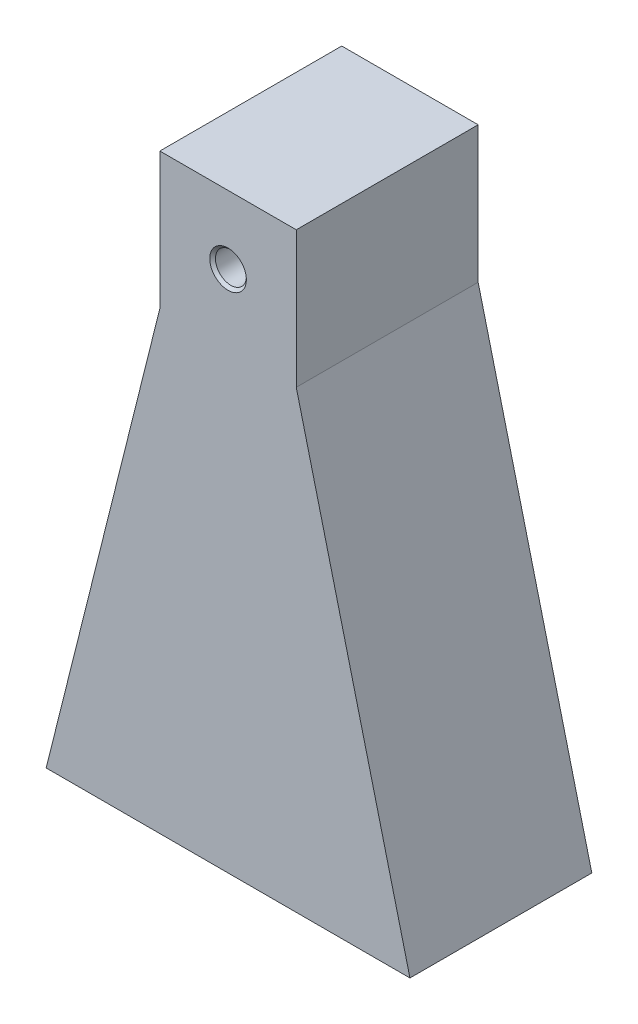
from build123d import *

# Parameters (mm, degrees)
BOSS_EXTRUDE1_DEPTH         = 40
M8_TAPPED_HOLE1_D           = 6.8
M8_TAPPED_HOLE1_CSINK_D     = 8.05
M8_TAPPED_HOLE1_CSINK_ANGLE = 90


with BuildPart() as part:
    # Sketch1 → Boss-Extrude1 (new body)
    with BuildSketch(Plane.XY):
        Polygon((40, -72.727272727), (-40, -72.727272727), (-15, 27.272727273), (-15, 57.272727273), (15, 57.272727273), (15, 27.272727273), align=None)
    extrude(amount=BOSS_EXTRUDE1_DEPTH)

    # M8 Tapped Hole1 (through all)
    with Locations(Plane.XY.offset(40)):
        with Locations((0, 42.272727273)):
            CounterSinkHole(M8_TAPPED_HOLE1_D / 2, M8_TAPPED_HOLE1_CSINK_D / 2, counter_sink_angle=M8_TAPPED_HOLE1_CSINK_ANGLE)


solid = part.part
